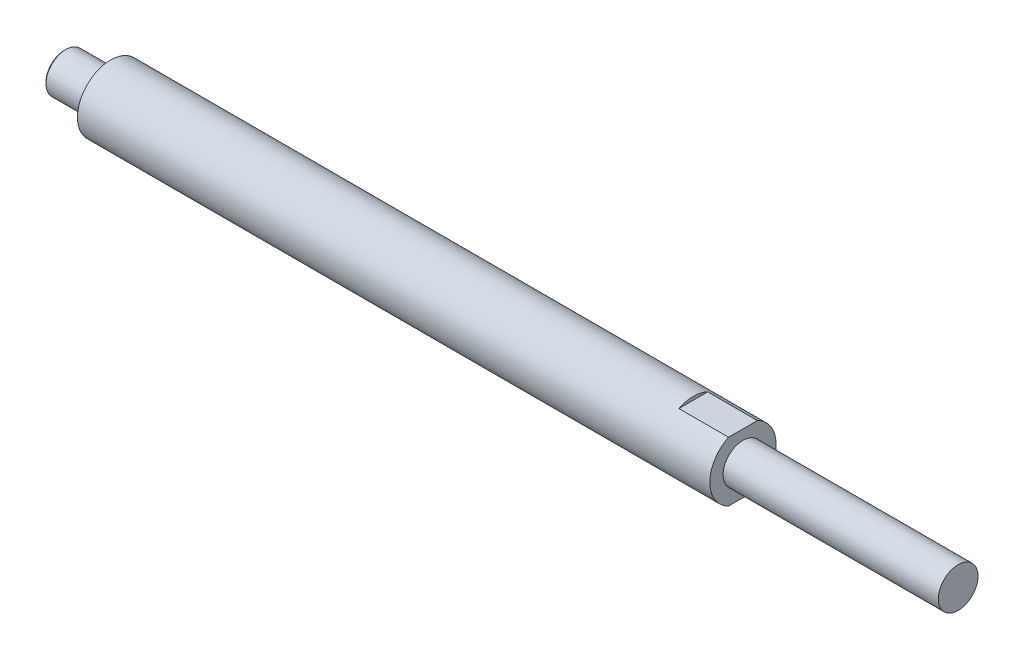
SolidWorks part; units mm, degrees
material "普通碳钢"
ref_plane "Front Plane" through (0, 0, 0) normal (0, 0, 1) x (1, 0, 0)
ref_plane "Top Plane" through (0, 0, 0) normal (0, 1, 0) x (1, 0, 0)
ref_plane "Right Plane" through (0, 0, 0) normal (1, 0, 0) x (0, 0, -1)
sketch "Sketch1" plane through (0, 0, 0) normal (0, 0, 1) x (1, 0, 0)
  line L0 (0, 0) -> (0, 10)
  line L3 (0, 10) -> (191, 10)
  line L4 (191, 10) -> (191, 6)
  line L5 (191, 6) -> (256, 6)
  line L6 (256, 6) -> (256, 0)
  line L7 (0, 0) -> (256, 0) construction
  line L8 (0, 0) -> (256, 0)
  dimension "D1" = 6
  dimension "D2" = 10
  dimension "D4" = 256
  dimension "D5" = 70
revolve "Revolve1" add sketch "Sketch1" angle 360 about L7
cosmetic thread "Cosmetic Thread1" parameters "D2"=10.106
sketch "Sketch6" plane through (0, 0, 0) normal (-1, 0, 0) x (0, 0, 1)
  circle A0 centre (0, 0) radius 6
  dimension "D1" = 12
extrude "Boss-Extrude1" add sketch "Sketch6" along normal blind 14
cosmetic thread "Cosmetic Thread2" parameters "D2"=10.106
chamfer "Chamfer1" distance 0.5 angle 45 1 edges at (-14, 0, 6)
sketch "Sketch7" plane through (0, 0, 0) normal (0, 0, 1) x (1, 0, 0)
  line L0 (191, 0) -> (136.9114, 0) construction
  line L2 (191, 10) -> (176, 10)
  line L7 (191, 10) -> (191, 9)
  line L8 (191, 9) -> (176, 9)
  line L9 (176, 10) -> (176, 9)
  line L10 (191, -6) -> (191, 6) construction
  line L11 (176, -10) -> (176, -9)
  line L12 (191, -9) -> (176, -9)
  line L13 (191, -10) -> (191, -9)
  line L14 (191, -10) -> (176, -10)
  dimension "D1" = 15
  dimension "D2" = 18
extrude "Cut-Extrude1" cut sketch "Sketch7" against normal mid plane 20
